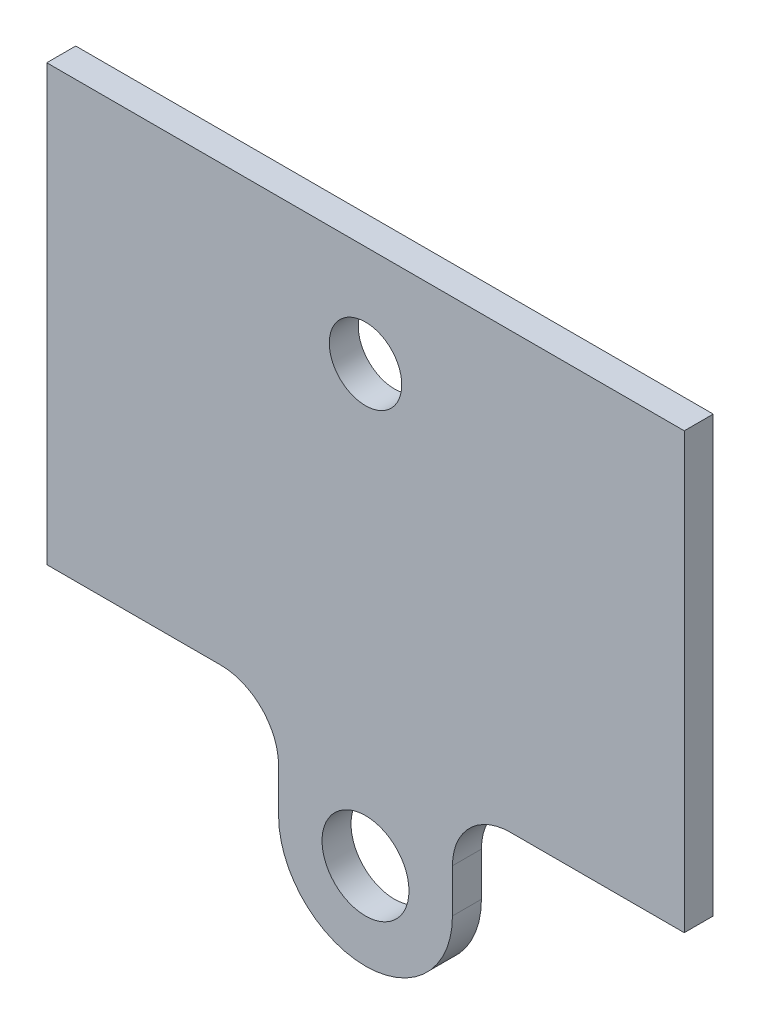
SolidWorks part; units mm, degrees
material "Q235B"
ref_plane "Front Plane" through (0, 0, 0) normal (0, 0, 1) x (1, 0, 0)
ref_plane "Top Plane" through (0, 0, 0) normal (0, 1, 0) x (1, 0, 0)
ref_plane "Right Plane" through (0, 0, 0) normal (1, 0, 0) x (0, 0, -1)
sketch "Sketch1" plane through (0, 0, 0) normal (0, 0, 1) x (1, 0, 0)
  line L0 (0, -75) -> (0, -110) construction
  line L1 (110, -75) -> (-110, -75)
  line L2 (110, -75) -> (110, 75)
  line L3 (110, 75) -> (-110, 75)
  line L4 (-110, -75) -> (-110, 75)
  line L5 (110, -75) -> (-110, 75) construction
  line L6 (110, 75) -> (-110, -75) construction
  line L7 (30, -75) -> (30, -110)
  line L8 (-30, -75) -> (-30, -110)
  line L9 (0, 40) -> (0, 75) construction
  arc A0 (30, -75) -> (-30, -75) centre (0, -75) ccw
  arc A1 (-30, -110) -> (30, -110) centre (0, -110) ccw
  circle A2 centre (0, -110) radius 15
  circle A3 centre (0, 40) radius 12.5
  point P0 (0, 0)
  point P8 (0, -92.5)
  dimension "D4" = 30
  dimension "D5" = 30
  dimension "D6" = 25
  dimension "D1" = 150
  dimension "D2" = 220
  dimension "D3" = 35
  dimension "D7" = 35
extrude "Boss-Extrude1" add sketch "Sketch1" along normal mid plane 10 contours L8 A1 L7 L1 A2 | A0 L1 L2 L3 L4 A3 | L1 A0
fillet "Fillet1" radius 20 2 edges at (-30, -75, 0) (30, -75, 0)
